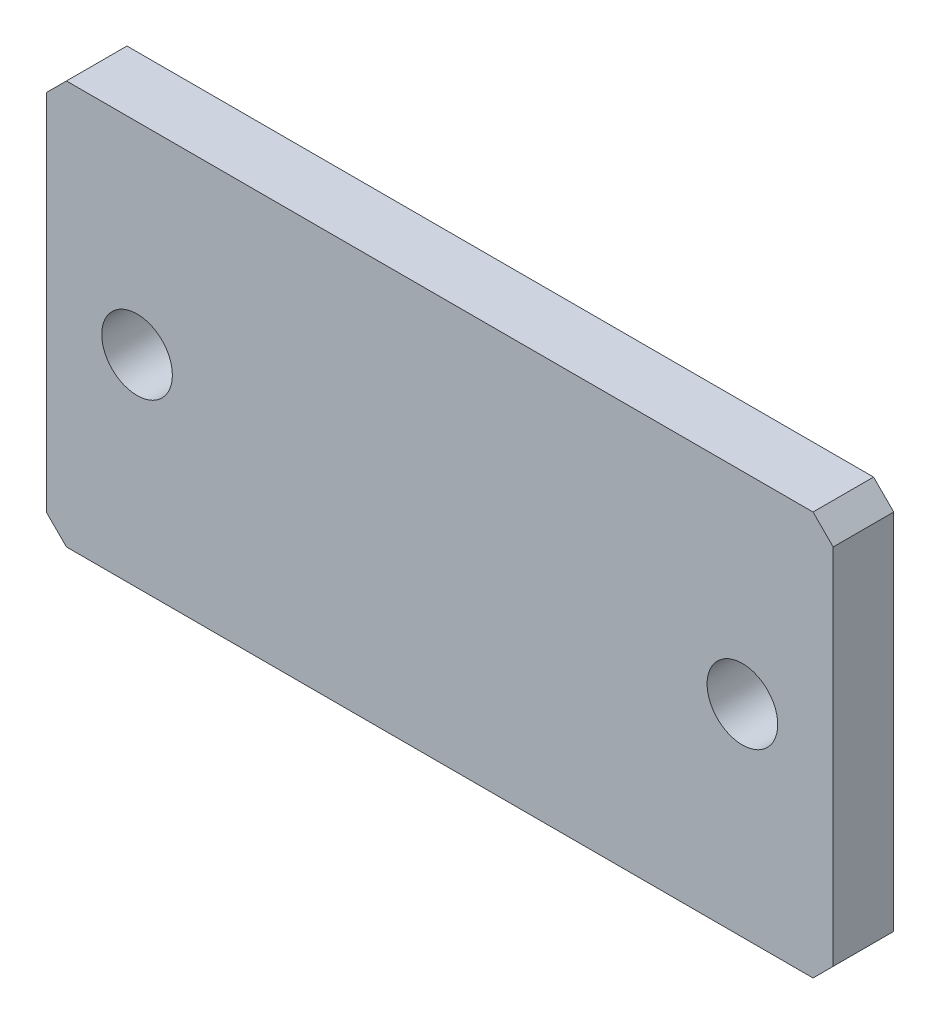
from build123d import *

# Parameters (mm, degrees)
SKETCH1_W           = 39
SKETCH1_H           = 20
SKETCH1_R           = 1.75
BOSS_EXTRUDE1_DEPTH = 3
CHAMFER1_SIZE       = 1


with BuildPart() as part:
    # Sketch1 → Boss-Extrude1 (new body)
    with BuildSketch(Plane.XY):
        Rectangle(SKETCH1_W, SKETCH1_H)
        with Locations((-15, 0)):
            Circle(SKETCH1_R, mode=Mode.SUBTRACT)
        with Locations((15, 0)):
            Circle(SKETCH1_R, mode=Mode.SUBTRACT)
    extrude(amount=BOSS_EXTRUDE1_DEPTH)

    # Chamfer1
    chamfer1_edges = [part.edges().sort_by_distance(p)[0] for p in [
        (19.5, -10, 1.5),
        (-19.5, -10, 1.5),
        (-19.5, 10, 1.5),
        (19.5, 10, 1.5),
    ]]
    chamfer(chamfer1_edges, length=CHAMFER1_SIZE)


solid = part.part
